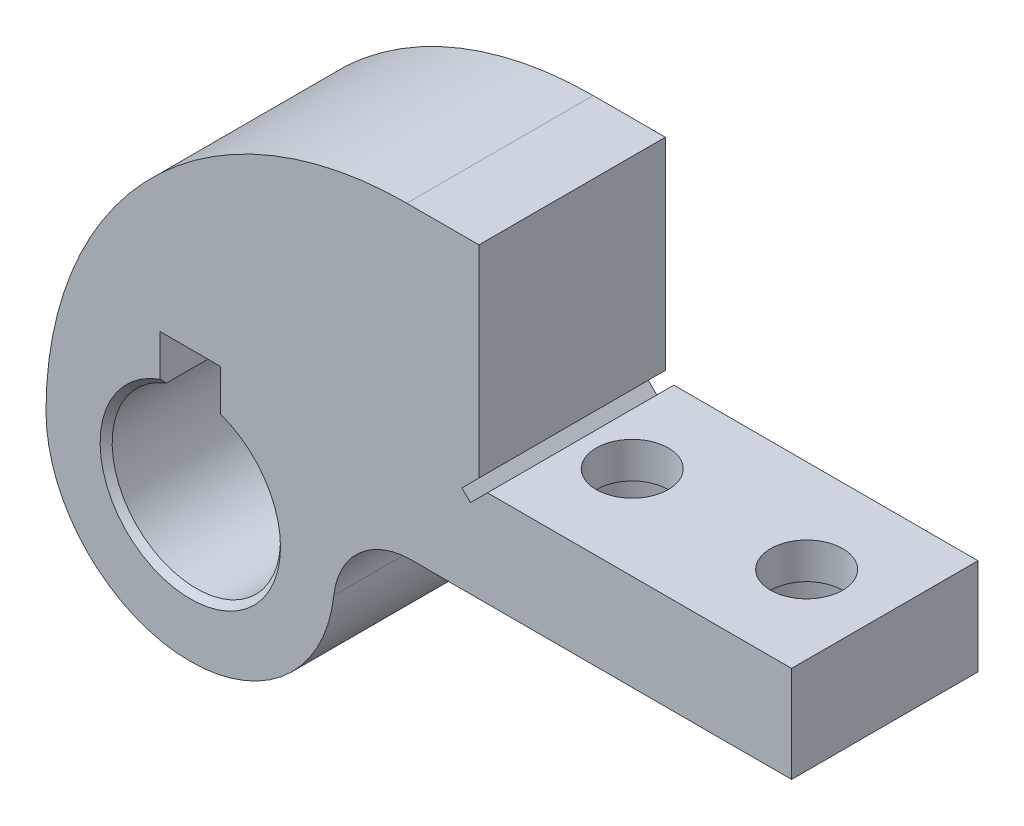
SolidWorks part; units mm, degrees
ref_plane "Front Plane" through (0, 0, 0) normal (0, 0, 1) x (1, 0, 0)
ref_plane "Top Plane" through (0, 0, 0) normal (0, 1, 0) x (1, 0, 0)
ref_plane "Right Plane" through (0, 0, 0) normal (1, 0, 0) x (0, 0, -1)
other "Configuration Table"
sketch "Sketch2" plane through (0, 0, 0) normal (0, 0, 1) x (1, 0, 0)
  line L0 (-21.5925, 0) -> (21.5925, 0) construction
  line L1 (18, 30) -> (24, 30)
  line L2 (24, 30) -> (24, 12.5)
  line L3 (24, 12.5) -> (50, 12.5)
  line L4 (50, 12.5) -> (50, 4.5)
  line L5 (50, 4.5) -> (18.3916, 4.5)
  line L7 (0, 11.1269) -> (0, 0) construction
  line L8 (-2.5, 6.5383) -> (-2.5, 10.5)
  line L9 (-2.5, 10.5) -> (2.5, 10.5)
  line L10 (0, 0) -> (0, -18.0848) construction
  line L11 (2.5, 6.5383) -> (2.5, 10.5)
  arc A0 (-2.5, 6.5383) -> (2.5, 6.5383) centre (0, 0) ccw
  arc A1 (11.9297, -1.2973) -> (-12, 0) centre (0, 0) cw
  arc A2 (-12, 0) -> (18, 30) centre (18, 0) cw
  arc A3 (18.3916, 4.5) -> (11.9297, -1.2973) centre (18.3916, -2) ccw
  point P20 (0, 10.5)
  dimension "D1" = 14
  dimension "D2" = 12
  dimension "D3" = 30
  dimension "D7" = 6.5
  dimension "D4" = 26
  dimension "D5" = 8
  dimension "D6" = 50
  dimension "D8" = 4.5
  dimension "D9" = 5
  dimension "D10" = 10.5
extrude "Boss-Extrude1" add sketch "Sketch2" along normal mid plane 15.5
sketch "Sketch3" plane through (0, 12.5, 0) normal (0, 1, 0) x (1, 0, 0)
  line L0 (0, 0) -> (29, 0) construction
  line L1 (29, 0) -> (43.5, 0) construction
  line L2 (50, -7.75) -> (50, 7.75) construction
  circle A0 centre (29, 0) radius 3
  circle A1 centre (43.5, 0) radius 3
  point P7 (29, 0)
  point P8 (43.5, 0)
  dimension "D3" = 6
  dimension "D4" = 6
  dimension "D1" = 6.5
  dimension "D2" = 14.5
extrude "Cut-Extrude1" cut sketch "Sketch3" against normal through all both and the other way through all
sketch "Sketch4" plane through (0, 4.5, 0) normal (0, -1, 0) x (1, 0, 0)
  circle A0 centre (29, 0) radius 5.25
  circle A1 centre (43.5, 0) radius 5.25
  dimension "D1" = 10.5
extrude "Cut-Extrude2" cut sketch "Sketch4" against normal blind 5
sketch "Sketch5" plane through (0, 0, 7.75) normal (0, 0, 1) x (1, 0, 0)
  line L0 (24, 13.2071) -> (22.5858, 11.7929)
  line L1 (24, 13.2071) -> (24.7071, 12.5)
  line L2 (22.5858, 11.7929) -> (23.2929, 11.0858)
  line L3 (24.3536, 12.8536) -> (22.9393, 11.4393) construction
  line L4 (24, 12.5) -> (24, 30) construction
  line L5 (24, 12.5) -> (21.026, 9.526) construction
  line L6 (50, 12.5) -> (24, 12.5) construction
  line L7 (24.7071, 12.5) -> (23.2929, 11.0858)
  dimension "D1" = 135
  dimension "D2" = 1
  dimension "D3" = 1.5
extrude "Cut-Extrude3" cut sketch "Sketch5" against normal through all both and the other way through all
chamfer "Chamfer2" distance 0.5 angle 45 2 edges at (0, -7, -7.75) (0, -7, 7.75)
